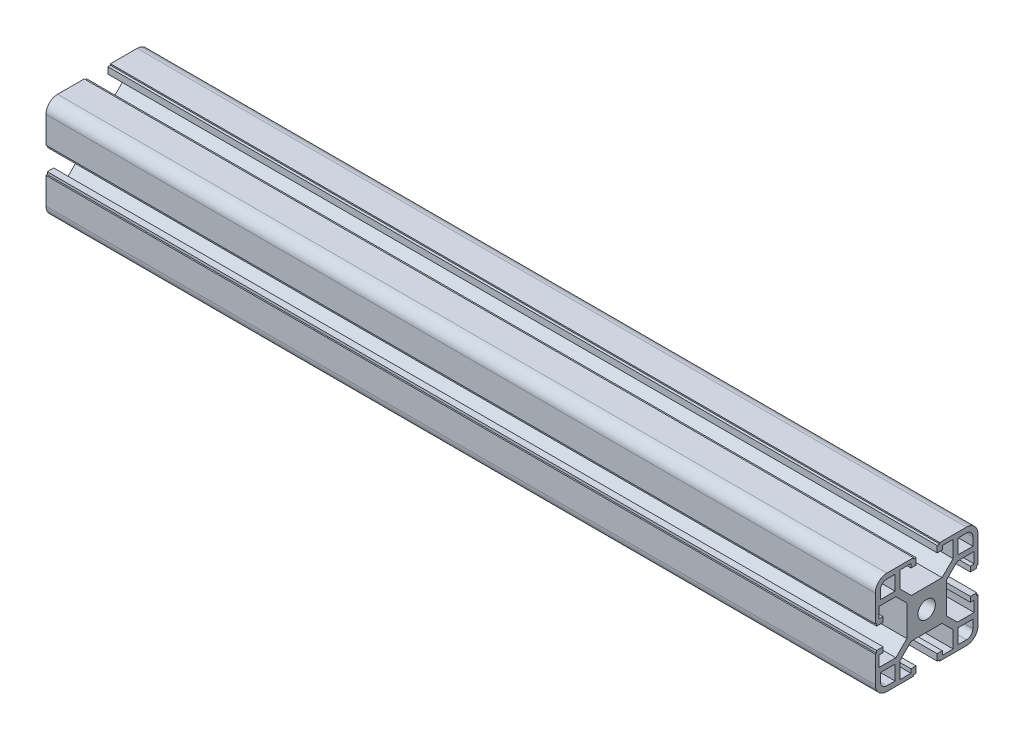
from build123d import *

# Parameters (mm, degrees)
SKETCH1_R                                 = 3.4
ALUMINIUM_PROFILE_40_X_40B_X_R4_5_1_DEPTH = 323


with BuildPart() as part:
    # Sketch1 → Aluminium profile 40 X 40B X R4.5(1) (new body)
    with BuildSketch(Plane.YZ.offset(-984.974958264)):
        with BuildLine():
            Line((-5.1, 20), (-5.1, 19.5))
            Line((-5.1, 19.5), (-4.1, 19.5))
            Line((-4.1, 19.5), (-4.1, 17))
            Line((-4.1, 17), (-6.1, 17))
            Line((-6.1, 17), (-6.1, 18.5))
            Line((-6.1, 18.5), (-10.3, 18.5))
            Line((-10.3, 18.5), (-10.3, 12))
            Line((-10.3, 12), (-6, 7.7))
            Line((-6, 7.7), (6, 7.7))
            Line((6, 7.7), (10.3, 12))
            Line((10.3, 12), (10.3, 18.5))
            Line((10.3, 18.5), (6.1, 18.5))
            Line((6.1, 18.5), (6.1, 17))
            Line((6.1, 17), (4.1, 17))
            Line((4.1, 17), (4.1, 19.5))
            Line((4.1, 19.5), (5.1, 19.5))
            Line((5.1, 19.5), (5.1, 20))
            Line((5.1, 20), (15.5, 20))
            ThreePointArc((15.5, 20), (18.681980515, 18.681980515), (20, 15.5))
            Line((20, 15.5), (20, 5.1))
            Line((20, 5.1), (19.5, 5.1))
            Line((19.5, 5.1), (19.5, 4.1))
            Line((19.5, 4.1), (17, 4.1))
            Line((17, 4.1), (17, 6.1))
            Line((17, 6.1), (18.5, 6.1))
            Line((18.5, 6.1), (18.5, 10.3))
            Line((18.5, 10.3), (12, 10.3))
            Line((12, 10.3), (7.7, 6))
            Line((7.7, 6), (7.7, -6))
            Line((7.7, -6), (12, -10.3))
            Line((12, -10.3), (18.5, -10.3))
            Line((18.5, -10.3), (18.5, -6.1))
            Line((18.5, -6.1), (17, -6.1))
            Line((17, -6.1), (17, -4.1))
            Line((17, -4.1), (19.5, -4.1))
            Line((19.5, -4.1), (19.5, -5.1))
            Line((19.5, -5.1), (20, -5.1))
            Line((20, -5.1), (20, -15.5))
            ThreePointArc((20, -15.5), (18.681980515, -18.681980515), (15.5, -20))
            Line((15.5, -20), (5.1, -20))
            Line((5.1, -20), (5.1, -19.5))
            Line((5.1, -19.5), (4.1, -19.5))
            Line((4.1, -19.5), (4.1, -17))
            Line((4.1, -17), (6.1, -17))
            Line((6.1, -17), (6.1, -18.5))
            Line((6.1, -18.5), (10.3, -18.5))
            Line((10.3, -18.5), (10.3, -12))
            Line((10.3, -12), (6, -7.7))
            Line((6, -7.7), (-6, -7.7))
            Line((-6, -7.7), (-10.3, -12))
            Line((-10.3, -12), (-10.3, -18.5))
            Line((-10.3, -18.5), (-6.1, -18.5))
            Line((-6.1, -18.5), (-6.1, -17))
            Line((-6.1, -17), (-4.1, -17))
            Line((-4.1, -17), (-4.1, -19.5))
            Line((-4.1, -19.5), (-5.1, -19.5))
            Line((-5.1, -19.5), (-5.1, -20))
            Line((-5.1, -20), (-15.5, -20))
            ThreePointArc((-15.5, -20), (-18.681980515, -18.681980515), (-20, -15.5))
            Line((-20, -15.5), (-20, -5.1))
            Line((-20, -5.1), (-19.5, -5.1))
            Line((-19.5, -5.1), (-19.5, -4.1))
            Line((-19.5, -4.1), (-17, -4.1))
            Line((-17, -4.1), (-17, -6.1))
            Line((-17, -6.1), (-18.5, -6.1))
            Line((-18.5, -6.1), (-18.5, -10.3))
            Line((-18.5, -10.3), (-12, -10.3))
            Line((-12, -10.3), (-7.7, -6))
            Line((-7.7, -6), (-7.7, 6))
            Line((-7.7, 6), (-12, 10.3))
            Line((-12, 10.3), (-18.5, 10.3))
            Line((-18.5, 10.3), (-18.5, 6.1))
            Line((-18.5, 6.1), (-17, 6.1))
            Line((-17, 6.1), (-17, 4.1))
            Line((-17, 4.1), (-19.5, 4.1))
            Line((-19.5, 4.1), (-19.5, 5.1))
            Line((-19.5, 5.1), (-20, 5.1))
            Line((-20, 5.1), (-20, 15.5))
            ThreePointArc((-20, 15.5), (-18.681980515, 18.681980515), (-15.5, 20))
            Line((-15.5, 20), (-5.1, 20))
        make_face()
        Circle(SKETCH1_R, mode=Mode.SUBTRACT)
        with BuildLine():
            Line((12.3, 18), (15.5, 18))
            ThreePointArc((15.5, 18), (17.267766953, 17.267766953), (18, 15.5))
            Line((18, 15.5), (18, 12.3))
            Line((18, 12.3), (12.3, 12.3))
            Line((12.3, 12.3), (12.3, 18))
        make_face(mode=Mode.SUBTRACT)
        with BuildLine():
            Line((-15.5, 18), (-12.3, 18))
            Line((-12.3, 18), (-12.3, 12.3))
            Line((-12.3, 12.3), (-18, 12.3))
            Line((-18, 12.3), (-18, 15.5))
            ThreePointArc((-18, 15.5), (-17.267766953, 17.267766953), (-15.5, 18))
        make_face(mode=Mode.SUBTRACT)
        with BuildLine():
            Line((-18, -12.3), (-12.3, -12.3))
            Line((-12.3, -12.3), (-12.3, -18))
            Line((-12.3, -18), (-15.5, -18))
            ThreePointArc((-15.5, -18), (-17.267766953, -17.267766953), (-18, -15.5))
            Line((-18, -15.5), (-18, -12.3))
        make_face(mode=Mode.SUBTRACT)
        with BuildLine():
            Line((12.3, -12.3), (18, -12.3))
            Line((18, -12.3), (18, -15.5))
            ThreePointArc((18, -15.5), (17.267766953, -17.267766953), (15.5, -18))
            Line((15.5, -18), (12.3, -18))
            Line((12.3, -18), (12.3, -12.3))
        make_face(mode=Mode.SUBTRACT)
    extrude(amount=ALUMINIUM_PROFILE_40_X_40B_X_R4_5_1_DEPTH)


solid = part.part
